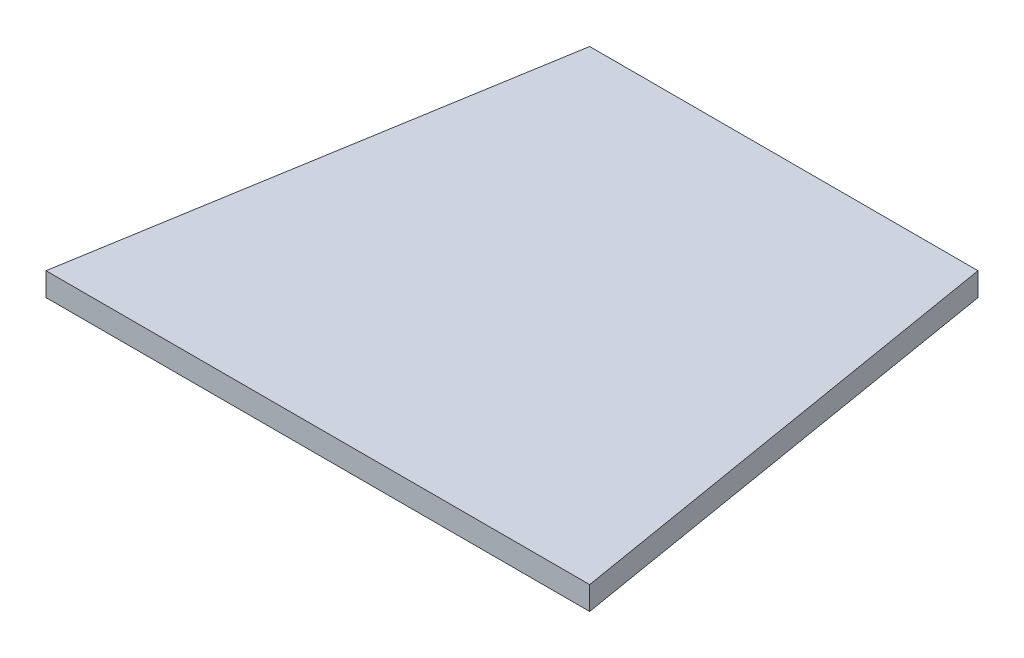
from build123d import *

# Parameters (mm, degrees)
BOSS_EXTRUDE1_DEPTH = 3


with BuildPart() as part:
    # Sketch1 → Boss-Extrude1 (new body)
    with BuildSketch(Plane(origin=(0, 0, 0), x_dir=(1, 0, 0), z_dir=(0, 1, 0))):
        Polygon((-25, 30), (25, 30), (35, -30), (-35, -30), align=None)
    extrude(amount=BOSS_EXTRUDE1_DEPTH)


solid = part.part
